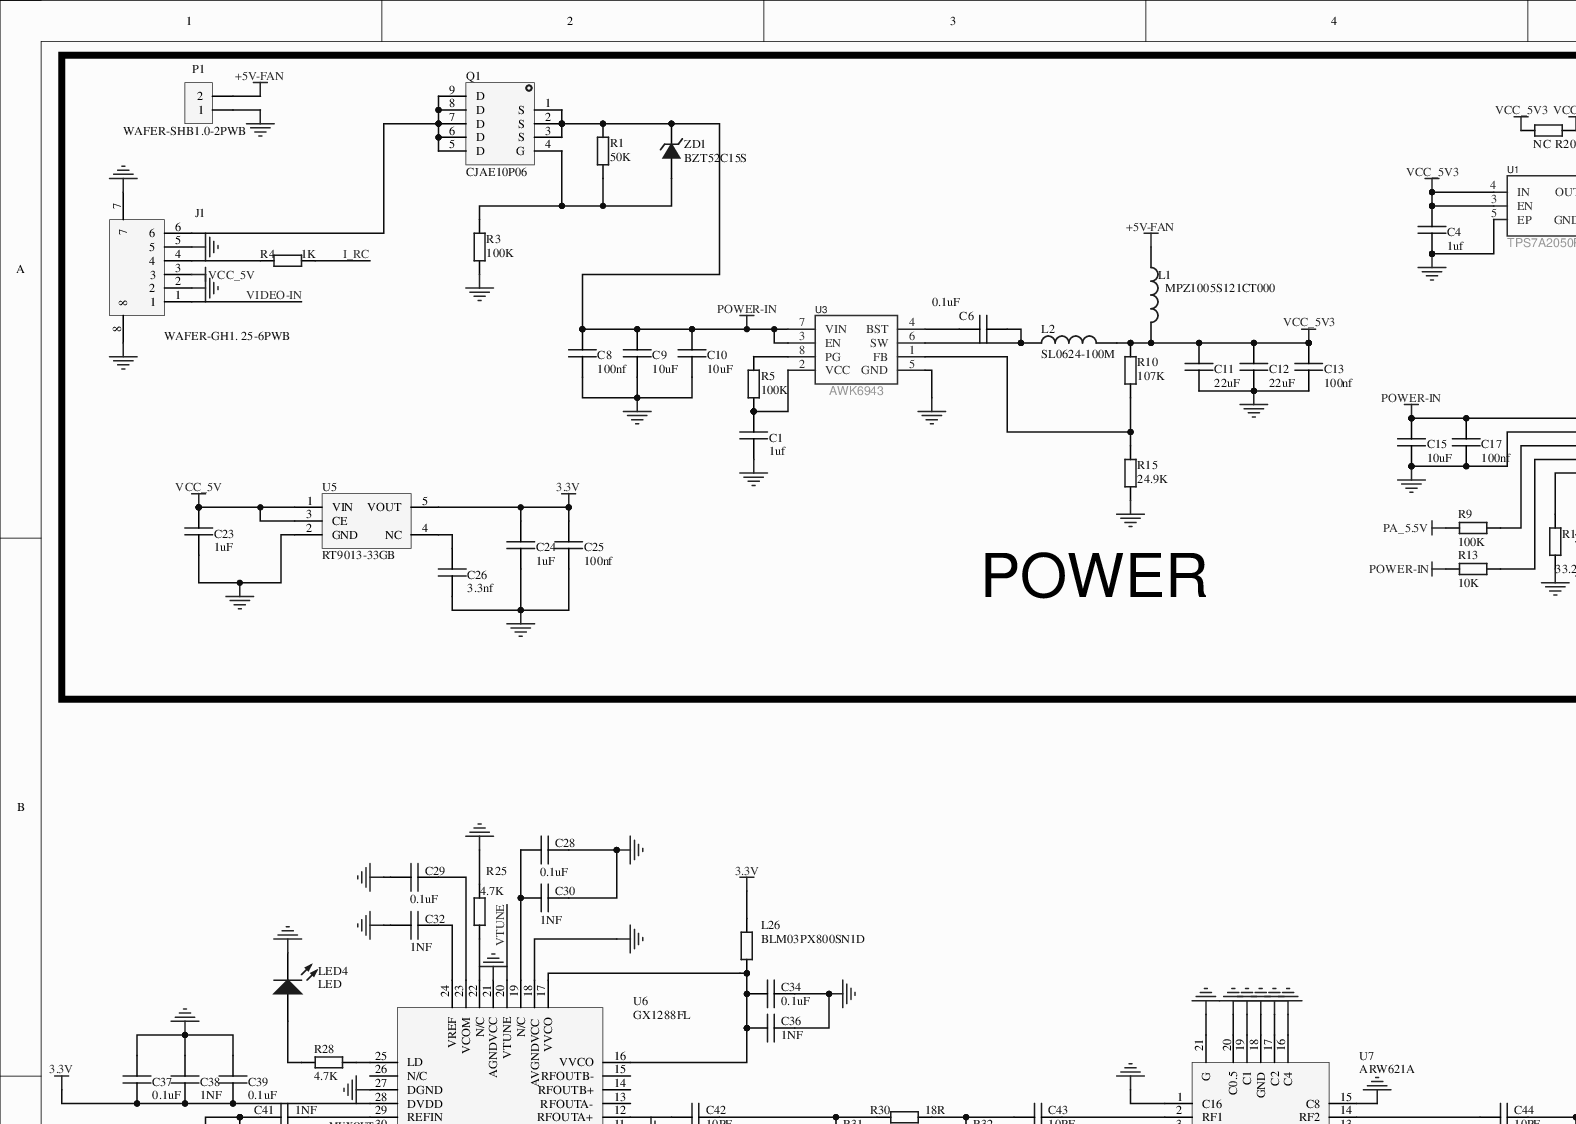
[diagram p0: MISC62792-2.SchDoc, top left]
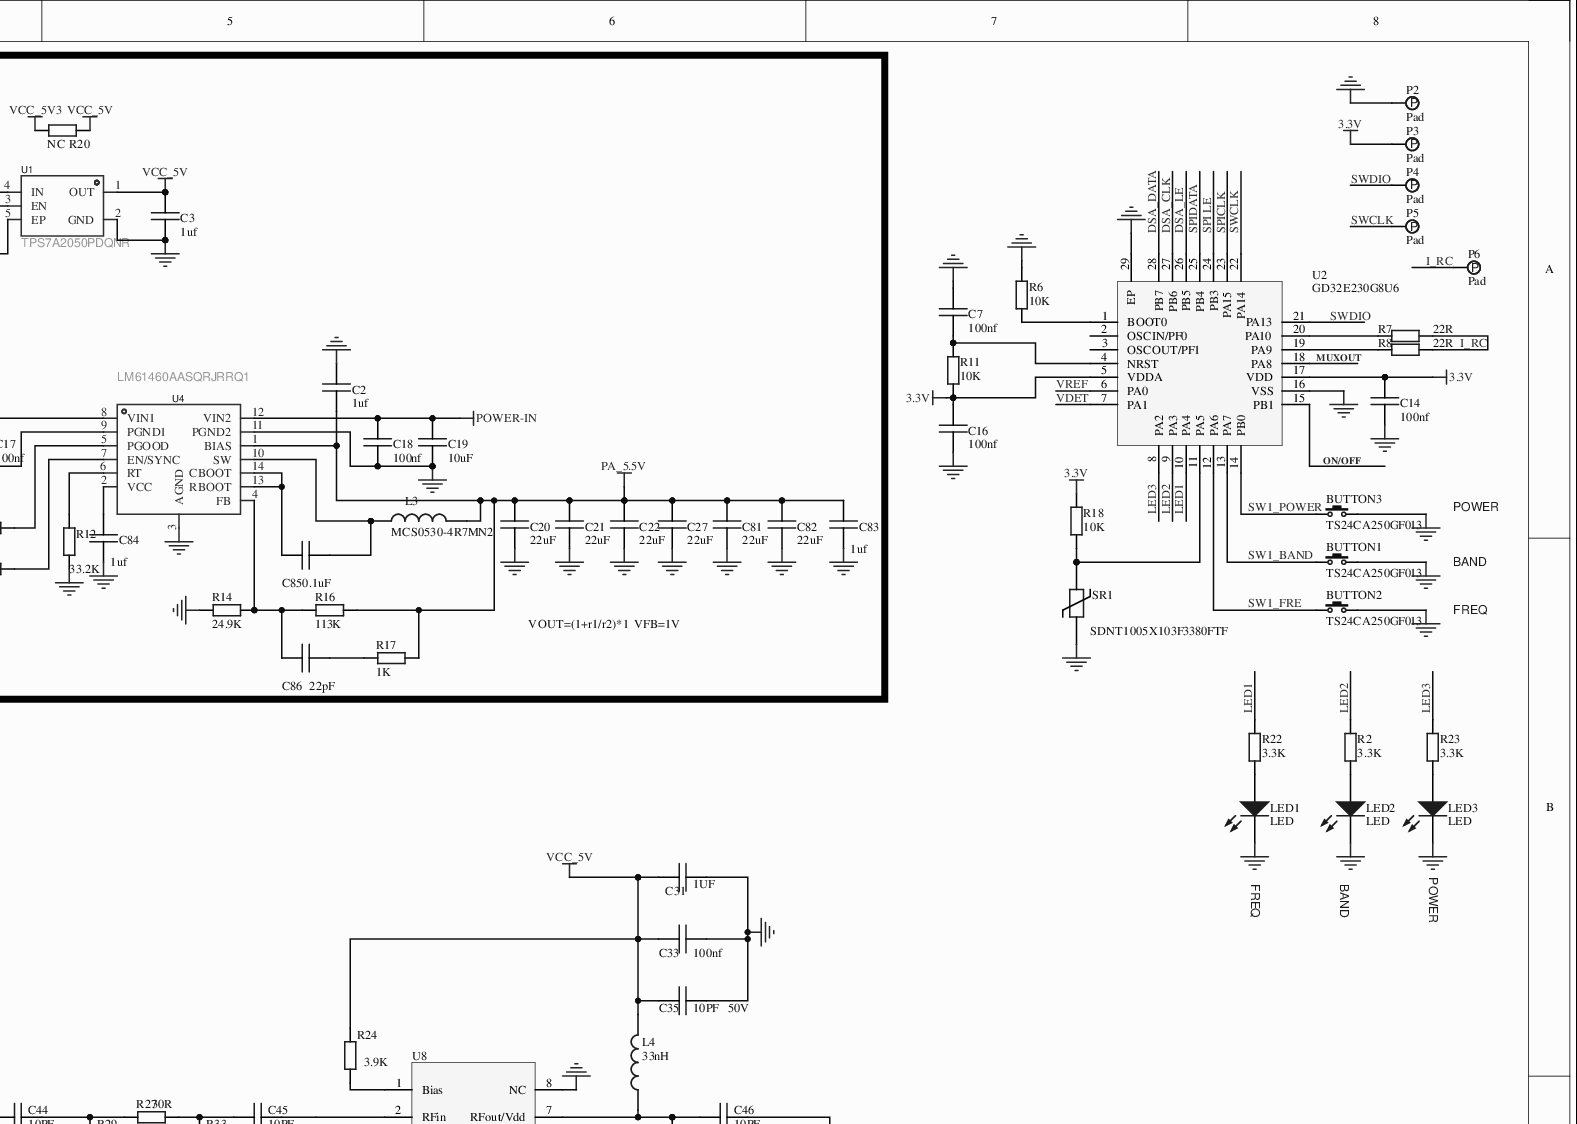
[diagram p1: MISC62792-2.SchDoc, top right]
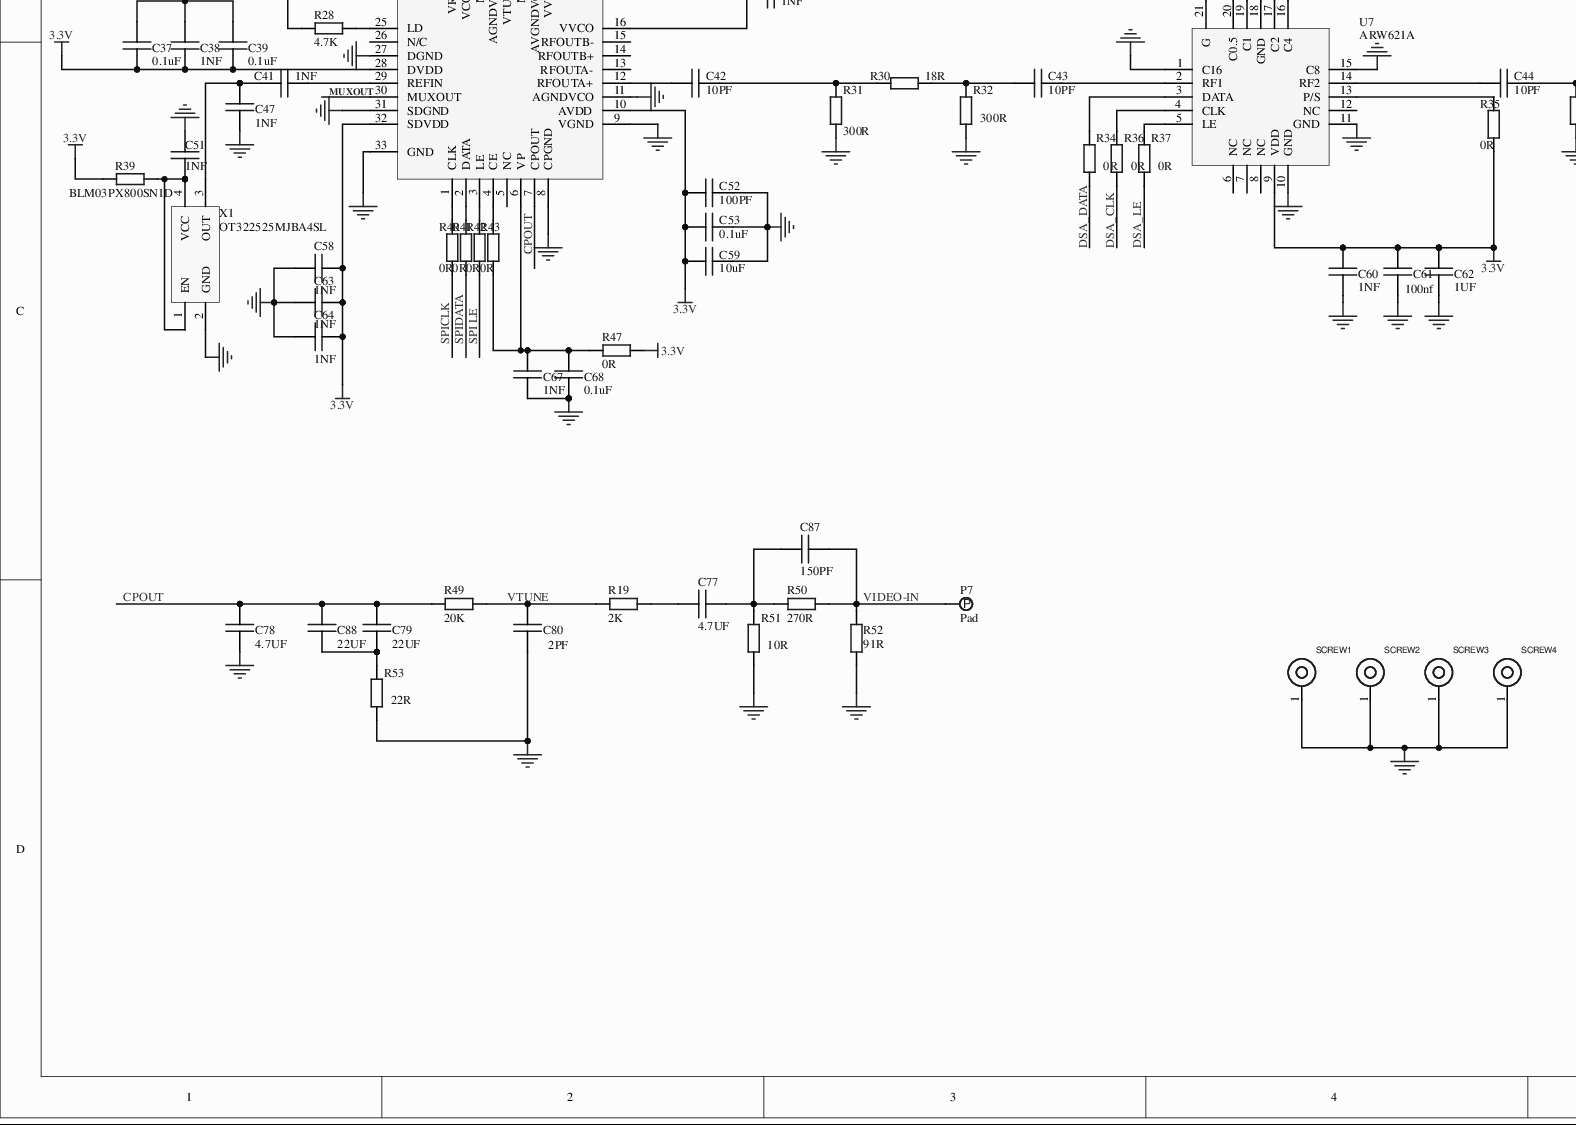
[diagram p2: MISC62792-2.SchDoc, bottom left]
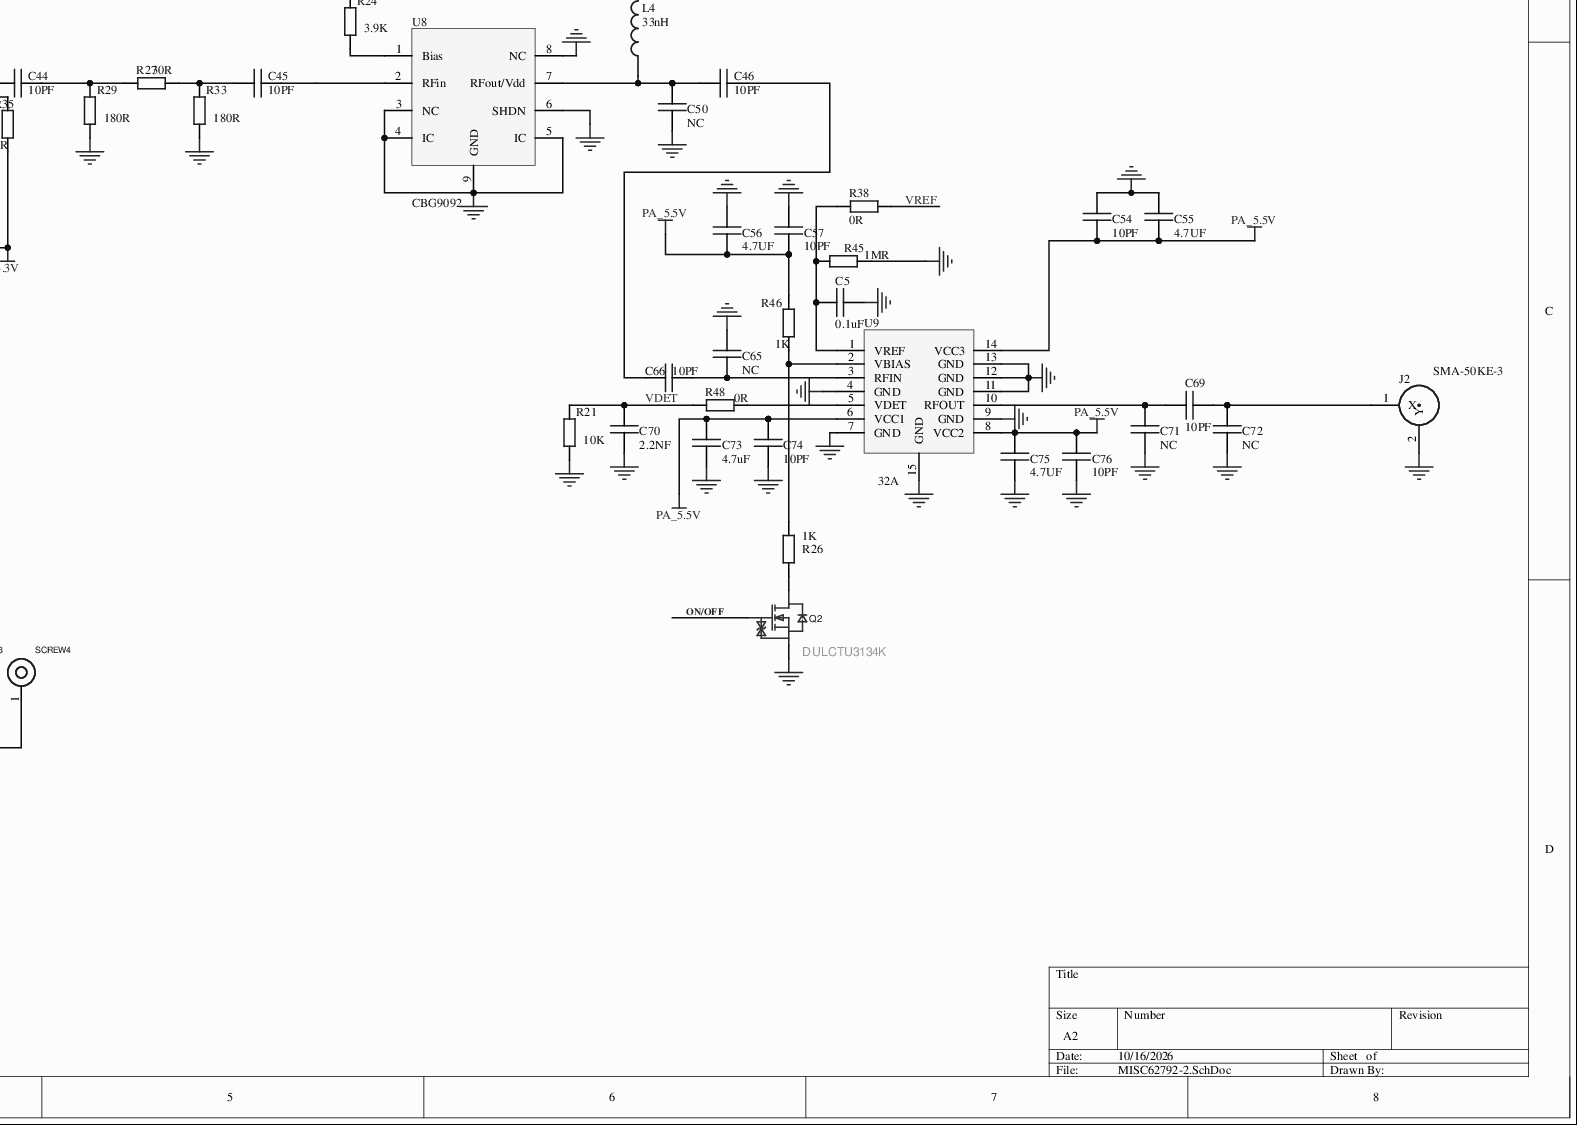
[diagram p3: MISC62792-2.SchDoc, bottom right]
# Altium project MISC62792-40.PrjPCB
1 sheet, 176 parts. Net scope: global (net labels, ports and power ports of the same name join across sheets).
Board file: MISC62792.PcbDoc

## Sheet MISC62792-2.SchDoc
size A2; SheetNumber: 1; SheetTotal: 1

### Parts
BUTTON1  TS24CA250GF013  [SW-SMD_L4.7-W3.5-P3.35-EH]
BUTTON2  TS24CA250GF013  [SW-SMD_L4.7-W3.5-P3.35-EH]
BUTTON3  TS24CA250GF013  [SW-SMD_L4.7-W3.5-P3.35-EH]
C1  1uf  [C0603]
C2  1uf  [C0603]
C3  1uf  [C0603]
C4  1uf  [C0603]
C5  0.1uF  [C0402]
C6  0.1uF  [C0402]
C7  100nf  [C0201]
C8  100nf  [C0402]
C9  10uF  [C0805]
C10  10uF  [C0805]
C11  22uF  [C0603]
C12  22uF  [C0603]
C13  100nf  [C0402]
C14  100nf  [C0201]
C15  10uF  [C0805]
C16  100nf  [C0201]
C17  100nf  [C0402]
C18  100nf  [C0402]
C19  10uF  [C0805]
C20  22uF  [C0603]
C21  22uF  [C0603]
C22  22uF  [C0603]
C23  1uF  [C0402]
C24  1uF  [C0402]
C25  100nf  [C0402]
C26  3.3nf  [C0402]
C27  22uF  [C0603]
C28  0.1uF  [C0201]
C29  0.1uF  [C0201]
C30  1NF  [C0201]
C31  1UF  [C0402]
C32  1NF  [C0201]
C33  100nf  [C0402]
C34  0.1uF  [C0201]
C35  10PF   50V  [C0402]
C36  1NF  [C0201]
C37  0.1uF  [C0201]
C38  1NF  [C0201]
C39  0.1uF  [C0201]
C41  1NF  [C0201]
C42  10PF  [C0402]
C43  10PF  [C0402]
C44  10PF  [C0402]
C45  10PF  [C0402]
C46  10PF  [C0402]
C47  1NF  [C0201]
C50  NC  [C0402]
C51  1NF  [C0201]
C52  100PF  [C0201]
C53  0.1uF  [C0201]
C54  10PF  [C0402]
C55  4.7UF  [C0603]
C56  4.7UF  [C0603]
C57  10PF  [C0402]
C58  1NF  [C0201]
C59  10uF  [C0402]
C60  1NF  [C0402]
C61  100nf  [C0402]
C62  1UF  [C0402]
C63  1NF  [C0201]
C64  1NF  [C0201]
C65  NC  [C0402]
C66  10PF  [C0402]
C67  1NF  [C0201]
C68  0.1uF  [C0201]
C69  10PF  [C0402]
C70  2.2NF  [C0402]
C71  NC  [C0402]
C72  NC  [C0402]
C73  4.7uF  [C0603]
C74  10PF  [C0402]
C75  4.7UF  [C0603]
C76  10PF  [C0402]
C77  4.7UF  [C0402]
C78  4.7UF  [C0402]
C79  22UF  [C0402]
C80  2PF  [C0402]
C81  22uF  [C0603]
C82  22uF  [C0603]
C83  1uf  [C0603]
C84  1uf  [C0603]
C85  0.1uF  [C0402]
C86  22pF  [C0402]
C87  150PF  [C0402]
C88  22UF  [C0402]
J1  WAFER-GH1. 25-6PWB  [SMD_6P-P1.25_XUNPU_WAFER-GH1.25-6PWB]
J2  SMA-50KE-3  [SMA-FP-945G]
L1  MPZ1005S121CT000  [L0402]
L2  SL0624-100M  [IND-SMD_L7.1-W6.6]
L3  MCS0530-4R7MN2  [IND-SMD_L5.2-W5.2_YSPI0530]
L4  33nH  [L0402]
L26  BLM03PX800SN1D  [L0201]
LED1  LED  [LED0402]
LED2  LED  [LED0402]
LED3  LED  [LED0402]
LED4  LED  [LED0402]
P1  WAFER-SHB1.0-2PWB  [SMD_2P-WAFER-SHB1.0-2PWB]
P2  Pad  [PAD]
P3  Pad  [PAD]
P4  Pad  [PAD]
P5  Pad  [PAD]
P6  Pad  [PAD]
P7  Pad  [PAD]
Q1  CJAE10P06  [DFN-8_L3.0-W3.0-P0.65-BL_G48N03D3]
Q2  DULCTU3134K  [SOT-523-3_L1.6-W0.8-P0.50-LS1.6-BR-1]
R1  50K  [R0402]
R2  3.3K  [R0402]
R3  100K  [R0402]
R4  1K  [R0402]
R5  100K  [R0402]
R6  10K  [R0201]
R7  22R  [R0201]
R8  22R  [R0201]
R9  100K  [R0402]
R10  107K  [R0402]
R11  10K  [R0201]
R12  33.2K  [R0402]
R13  10K  [R0402]
R14  24.9K  [R0402]
R15  24.9K  [R0402]
R16  113K  [R0402]
R17  1K  [R0402]
R18  10K  [R0201]
R19  2K  [R0402]
R20  NC  [R0402]
R21  10K  [R0402]
R22  3.3K  [R0402]
R23  3.3K  [R0402]
R24  3.9K  [R0402]
R25  4.7K  [R0201]
R26  1K  [R0402]
R27  30R  [R0402]
R28  4.7K  [R0201]
R29  180R  [R0402]
R30  18R  [R0402]
R31  300R  [R0402]
R32  300R  [R0402]
R33  180R  [R0402]
R34  0R  [R0402]
R35  0R  [R0402]
R36  0R  [R0402]
R37  0R  [R0402]
R38  0R  [R0402]
R39  BLM03PX800SN1D  [L0201]
R40  0R  [R0201]
R41  0R  [R0201]
R42  0R  [R0201]
R43  0R  [R0201]
R45  1MR  [R0402]
R46  1K  [R0402]
R47  0R  [R0201]
R48  0R  [R0402]
R49  20K  [R0402]
R50  270R  [R0402]
R51  10R  [R0402]
R52  91R  [R0402]
R53  22R  [R0402]
SCREW1  MARK_4  [M2]  (value not drawn)
SCREW2  MARK_4  [M2]  (value not drawn)
SCREW3  MARK_4  [M2]  (value not drawn)
SCREW4  MARK_4  [M2]  (value not drawn)
SR1  SDNT1005X103F3380FTF  [R0402]
U1  TPS7A2050PDQNR  [X2SON-4_L1.0-W1.0-P0.65-TL-EP]
U2  GD32E230G8U6  [QFN-28_L4.0-W4.0-P0.40-BL-EP2.8]
U3  AWK6943  [QFN-8_L3.0-W3.0-P0.65-BL]
U4  LM61460AASQRJRRQ1  [VQFN-14-HR_L4.0-W3.5-TL_LM61460AASQRJRRQ1]
U5  RT9013-33GB  [SOT-23-5_L3.0-W1.7-P0.95-LS2.8-BL]
U6  GX1288FL  [QFN-32_L5.0-W5.0-P0.50]
U7  ARW621A  [QFN-20_L4.0-W4.0-P0.50-TL-EP2.2]
U8  CBG9092  [CBG9092]
U9  32A  [AU64XX]
X1  OT322525MJBA4SL  [SMD3225]
ZD1  BZT52C15S  [SOD-323_L1.7-W1.3-LS2.6-RD]

### Blocks framed on the sheet
POWER: C1-C4 C6 C8-C13 C15 C17-C27 C81-C86 J1 L1-L3 P1 Q1 R1 R3-R5 R9 R10 R12-R17 R20 U1 U3-U5 ZD1

### Nets
3.3V: C14.1 C16.1 C24.1 C25.1 C37.2 C38.1 C39.2 C52.1 C53.2 C58.2 C59.2 C60.2 C61.2 C62.2 C63.2 C64.1 L26.1 P3.1 R11.2 R18.1 R35.2 R39.1 R47.2 U2.5(VDDA) U2.17(VDD) U5.5(VOUT) U6.10(AVDD) U6.28(DVDD) U6.32(SDVDD) U7.9(VDD)
+5V-FAN: L1.1 P1.2
GND: BUTTON1.1 BUTTON2.1 BUTTON3.1 C1.2 C2.2 C3.2 C4.2 C5.1 C7.1 C8.2 C9.2 C10.2 C11.2 C12.2 C13.2 C14.2 C15.2 C16.2 C17.2 C18.2 C19.2 C20.2 C21.2 C22.2 C23.2 C24.2 C25.2 C26.2 C27.2 C28.1 C29.2 C30.2 C31.1 C32.1 C33.1 C34.1 C35.2 C36.2 C37.1 C38.2 C39.1 C47.2 C50.2 C51.1 C52.2 C53.1 C54.2 C55.2 C56.1 C57.1 C58.1 C59.1 C60.1 C61.1 C62.1 C63.1 C64.2 C65.2 C67.2 C68.1 C70.1 C71.1 C72.1 C73.2 C74.2 C75.2 C76.2 C78.2 C80.1 C81.2 C82.2 C83.2 C84.2 J1.2 J1.5 J1.7 J1.8 J2.2(Y) LED1.2(K) LED2.2(K) LED3.2(K) LED4.2(K) P1.1 P2.1 Q2.2(S) R3.1 R6.1 R12.2 R14.2 R15.2 R21.2 R25.1 R29.2 R31.2 R32.2 R33.2 R45.2 R51.2 R52.2 R53.2 SCREW1.1 SCREW2.1 SCREW3.1 SCREW4.1 SR1.2 U1.2(GND) U1.5(EP) U2.16(VSS) U2.29(EP) U3.5(GND) U4.3(AGND) U4.9(PGND1) U4.11(PGND2) U5.2(GND) U6.8(CPGND) U6.9(VGND) U6.11(AGNDVCO) U6.18(AVGNDVCC) U6.21(AGNDVCC) U6.27(DGND) U6.31(SDGND) U6.33(GND) U7.1(C16) U7.10(GND) U7.11(GND) U7.15(C8) U7.16(C4) U7.17(C2) U7.18(GND) U7.19(C1) U7.20(C0.5) U7.21(G) U8.3(NC) U8.4(IC) U8.5(IC) U8.6(SHDN) U8.8(NC) U8.9(GND) U9.4(GND) U9.7(GND) U9.9(GND) U9.11(GND) U9.12(GND) U9.13(GND) U9.15(GND) X1.2(GND)
PA_5.5V: C2.1 C20.1 C21.1 C22.1 C27.1 C54.1 C55.1 C56.2 C57.2 C73.1 C74.1 C75.1 C76.1 C81.1 C82.1 C83.1 L3.2 R9.2 R16.1 R17.1 R46.1 U4.1(BIAS) U9.6(VCC1) U9.8(VCC2) U9.14(VCC3)
POWER-IN: C8.1 C9.1 C10.1 C15.1 C17.1 C18.1 C19.1 Q1.1(S) Q1.2(S) Q1.3(S) R1.2 R13.2 U3.3(EN) U3.7(VIN) U4.8(VIN1) U4.12(VIN2) ZD1.2(K)
VCC_5V: C3.1 C23.1 C31.2 C33.2 C35.1 J1.3 L4.2 R20.1 R24.1 U1.1(OUT) U5.1(VIN) U5.3(CE)
VCC_5V3: C4.1 C11.1 C12.1 C13.1 L1.2 L2.2 R10.1 R20.2 U1.3(EN) U1.4(IN)
CPOUT: C78.1 C79.2 C88.2 R49.1 U6.7(CPOUT)
DSA_CLK: R36.2 U2.27(PB6)
DSA_DATA: R34.2 U2.28(PB7)
DSA_LE: R37.2 U2.26(PB5)
I_RC: P6.1 R4.2 R7.2 R8.2
LED1: R22.1 U2.10(PA4)
LED2: R2.1 U2.9(PA3)
LED3: R23.1 U2.8(PA2)
MUXOUT: U2.18(PA8) U6.30(MUXOUT)
ON/OFF: Q2.1(G) U2.15(PB1)
SPI LE: R42.2 U2.24(PB3)
SPICLK: R40.2 U2.23(PA15)
SPIDATA: R41.2 U2.25(PB4)
SW1_BAND: BUTTON1.2 U2.13(PA7)
SW1_FRE: BUTTON2.2 U2.12(PA6)
SW1_POWER: BUTTON3.2 U2.14(PB0)
SWCLK: P5.1 U2.22(PA14)
SWDIO: P4.1 U2.21(PA13)
VDET: C70.2 R21.1 R48.1 U2.7(PA1)
VIDEO-IN: C87.1 J1.1 P7.1 R50.2 R52.1
VREF: R38.1 U2.6(PA0)
VTUNE: C80.2 R19.1 R49.2 U6.20(VTUNE)
NetC1_1: C1.1 R5.1 U3.2(VCC)
NetC5_2: C5.2 R38.2 R45.1 U9.1(VREF)
NetC6_1: C6.1 U3.4(BST)
NetC6_2: C6.2 L2.1 U3.6(SW)
NetC7_2: C7.2 R11.1 U2.4(NRST)
NetC26_1: C26.1 U5.4(NC)
NetC28_2: C28.2 C30.1 U6.19(N/C)
NetC29_1: C29.1 U6.23(VCOM)
NetC32_2: C32.2 U6.24(VREF)
NetC34_2: C34.2 C36.1 L26.2 U6.16(VVCO) U6.17(VVCO)
NetC41_1: C41.1 U6.29(REFIN)
NetC41_2: C41.2 C47.1 X1.3(OUT)
NetC42_1: C42.1 U6.12(RFOUTA+)
NetC42_2: C42.2 R30.1 R31.1
NetC43_1: C43.1 R30.2 R32.1
NetC43_2: C43.2 U7.2(RF1)
NetC44_1: C44.1 U7.14(RF2)
NetC44_2: C44.2 R27.1 R29.1
NetC45_1: C45.1 R27.2 R33.1
NetC45_2: C45.2 U8.2(RFin)
NetC46_1: C46.1 C50.1 L4.1 U8.7(RFout/Vdd)
NetC46_2: C46.2 C66.2
NetC51_2: C51.2 R39.2 X1.1(EN) X1.4(VCC)
NetC65_1: C65.1 C66.1 U9.3(RFIN)
NetC67_1: C67.1 C68.2 R43.2 R47.1 U6.6(VP)
NetC69_1: C69.1 C71.2 U9.10(RFOUT)
NetC69_2: C69.2 C72.2 J2.1(X)
NetC77_1: C77.1 C87.2 R50.1 R51.1
NetC77_2: C77.2 R19.2
NetC79_1: C79.1 C88.1 R53.1
NetC84_1: C84.1 U4.2(VCC)
NetC85_1: C85.1 U4.13(RBOOT) U4.14(CBOOT)
NetC85_2: C85.2 L3.1 U4.10(SW)
NetC86_1: C86.1 R14.1 R16.2 U4.4(FB)
NetC86_2: C86.2 R17.2
NetJ1_4: J1.4 R4.1
NetJ1_6: J1.6 Q1.5(D) Q1.6(D) Q1.7(D) Q1.8(D) Q1.9(D)
NetLED1_1: LED1.1(A) R22.2
NetLED2_1: LED2.1(A) R2.2
NetLED3_1: LED3.1(A) R23.2
NetLED4_1: LED4.1(A) R28.1
NetQ1_4: Q1.4(G) R1.1 R3.2 ZD1.1(A)
NetQ2_3: Q2.3(D) R26.2
NetR5_2: R5.2 U3.8(PG)
NetR6_2: R6.2 U2.1(BOOT0)
NetR7_1: R7.1 U2.20(PA10)
NetR8_1: R8.1 U2.19(PA9)
NetR9_1: R9.1 U4.5(PGOOD)
NetR10_2: R10.2 R15.1 U3.1(FB)
NetR12_1: R12.1 U4.6(RT)
NetR13_1: R13.1 U4.7(EN/SYNC)
NetR18_2: R18.2 SR1.1 U2.11(PA5)
NetR24_2: R24.2 U8.1(Bias)
NetR25_2: R25.2 U6.22(N/C)
NetR26_1: R26.1 R46.2 U9.2(VBIAS)
NetR28_2: R28.2 U6.25(LD)
NetR34_1: R34.1 U7.3(DATA)
NetR35_1: R35.1 U7.13(P/S)
NetR36_1: R36.1 U7.4(CLK)
NetR37_1: R37.1 U7.5(LE)
NetR40_1: R40.1 U6.1(CLK)
NetR41_1: R41.1 U6.2(DATA)
NetR42_1: R42.1 U6.3(LE)
NetR43_1: R43.1 U6.4(CE)
NetR48_2: R48.2 U9.5(VDET)

Not connected (* = marked no-connect by the designer): U2 2(OSCIN/PF0) 3(OSCOUT/PF1); U6 5(NC) 13(RFOUTA-) 14(RFOUTB+) 15(RFOUTB-) 26(N/C); U7 6(NC) 7(NC) 8(NC) 12(NC)

### Notes on the sheet
- POWER
- BAND
- VOUT=(1+r1/r2)*1  VFB=1V
- FREQ

### Library data of the parts
BUTTON1-BUTTON3 = TSW 3x6: 3x6 tactile switch; BOM名称: 3x6 tactile switch
C1-C6 C9-C12 C15 C19-C24 C26-C32 C34-C39 C41-C47 C50-C60 C62-C88 = 100nf
L1-L4 = L-AL: Color-ring inductor; BOM名称: Color-ring inductor
L26 R1-R43 R45-R53 = R: SMD resistor; 版权归属: From; BOM名称: SMD resistor
LED1-LED4 = LED0: Published: 8-Jun-2000; LatestRevisionDate: 08-Jul-2005; LatestRevisionNote: Mech Layer 1 removed.; PackageReference: LED-0; Publisher: Altium Limited
P1 = Header 2: 2P connector; BOM名称: 2P connector
Q2 = 2N7002T_C5224243: Symbol: 2N7002T_C5224243
SCREW1-SCREW4 = MARK_4: MARK Symble; RK_PN: MARK01; Priority: A; Created_by: CZD; Source_Path: RK3399_BOX_SCH_V1.0_20180521.DSN; Value: SCREEW; Part_Type: MARK; PCB DECAL: MARK
U3 = TPS54327DDAR: Symbol: TPS54327DDAR
U9 = GCM3527(3.3G-3.8G)
X1 = XTAL-ACT-4P: 4-pin active crystal oscillator; 版权归属: COMPANY_C; BOM名称: 4-pin active crystal oscillator
ZD1 = 1N4733: 5.1V/1W Zener diode; BOM名称: 5.1V/1W Zener diode
U1 = TPS7A2050PDQNR: Symbol: TPS7A2050PDQNR
U4 = LM61460AASQRJRRQ1: Symbol: LM61460AASQRJRRQ1